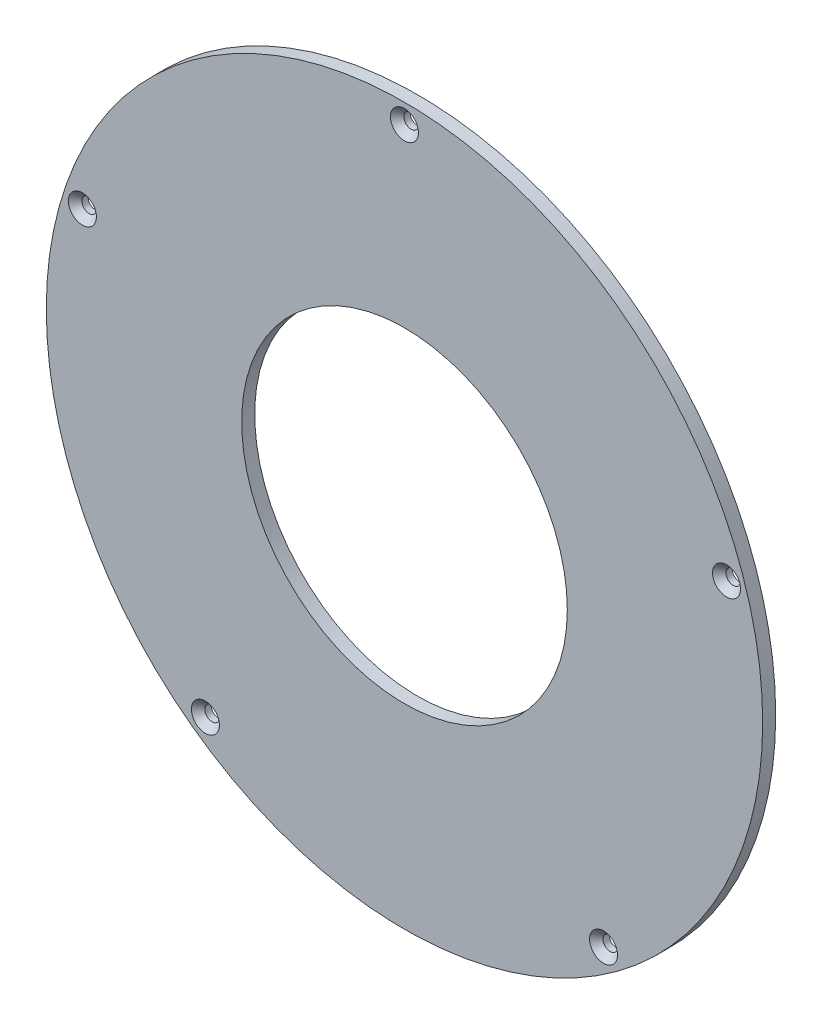
from build123d import *

# Parameters (mm, degrees)
SKETCH1_R                                 = 110
SKETCH1_R_2                               = 50
BOSS_EXTRUDE1_DEPTH                       = 4
HOLE_SIZE_PER_CROSS_SLOTTED_COUNT_2_COUNT = 2
HOLE_SIZE_PER_CROSS_SLOTTED_COUNT_2_PITCH = 122.259332477
HOLE_SIZE_PER_CROSS_SLOTTED_COUNT_3_COUNT = 2
HOLE_SIZE_PER_CROSS_SLOTTED_COUNT_3_PITCH = 197.819755389
HOLE_SIZE_PER_CROSS_SLOTTED_COUNT_4_COUNT = 2
HOLE_SIZE_PER_CROSS_SLOTTED_COUNT_4_PITCH = 197.819755389
HOLE_SIZE_PER_CROSS_SLOTTED_COUNT_5_COUNT = 2
HOLE_SIZE_PER_CROSS_SLOTTED_COUNT_5_PITCH = 122.259332477


with BuildPart() as part:
    # Sketch1 → Boss-Extrude1 (new body)
    with BuildSketch(Plane.XY):
        Circle(SKETCH1_R)
        Circle(SKETCH1_R_2, mode=Mode.SUBTRACT)
    extrude(amount=BOSS_EXTRUDE1_DEPTH)

    # Sketch5 → Hole Size (% per cross) Slotted Countersunk Wood Screw Type1 (revolve, cut)
    with BuildSketch(Plane(origin=(0, 104, 4), x_dir=(0, -1, 0), z_dir=(1, 0, 0))):
        Polygon((0, 0), (0, 4), (2.25, 4), (2.25, 2.05), (4.3, 0), align=None)
    hole_size_per_cross_slotted_countersu = revolve(axis=Axis((0, 104, 10.35), (0, 0, -1)), mode=Mode.SUBTRACT)

    # Hole Size _ per cross_ Slotted Count 2: Hole Size (% per cross) Slotted Countersunk Wood Screw Type1 ×2
    with Locations(*[Vector(0.8090169943749717, -0.5877852522924399, 0) * (i * HOLE_SIZE_PER_CROSS_SLOTTED_COUNT_2_PITCH) for i in range(1, HOLE_SIZE_PER_CROSS_SLOTTED_COUNT_2_COUNT)]):
        add(hole_size_per_cross_slotted_countersu, mode=Mode.SUBTRACT)

    # Hole Size _ per cross_ Slotted Count 3: Hole Size (% per cross) Slotted Countersunk Wood Screw Type1 ×2
    with Locations(*[Vector(0.3090169943749865, -0.9510565162951409, 0) * (i * HOLE_SIZE_PER_CROSS_SLOTTED_COUNT_3_PITCH) for i in range(1, HOLE_SIZE_PER_CROSS_SLOTTED_COUNT_3_COUNT)]):
        add(hole_size_per_cross_slotted_countersu, mode=Mode.SUBTRACT)

    # Hole Size _ per cross_ Slotted Count 4: Hole Size (% per cross) Slotted Countersunk Wood Screw Type1 ×2
    with Locations(*[Vector(-0.30901699437490837, -0.9510565162951663, 0) * (i * HOLE_SIZE_PER_CROSS_SLOTTED_COUNT_4_PITCH) for i in range(1, HOLE_SIZE_PER_CROSS_SLOTTED_COUNT_4_COUNT)]):
        add(hole_size_per_cross_slotted_countersu, mode=Mode.SUBTRACT)

    # Hole Size _ per cross_ Slotted Count 5: Hole Size (% per cross) Slotted Countersunk Wood Screw Type1 ×2
    with Locations(*[Vector(-0.8090169943749234, -0.5877852522925062, 0) * (i * HOLE_SIZE_PER_CROSS_SLOTTED_COUNT_5_PITCH) for i in range(1, HOLE_SIZE_PER_CROSS_SLOTTED_COUNT_5_COUNT)]):
        add(hole_size_per_cross_slotted_countersu, mode=Mode.SUBTRACT)


solid = part.part
